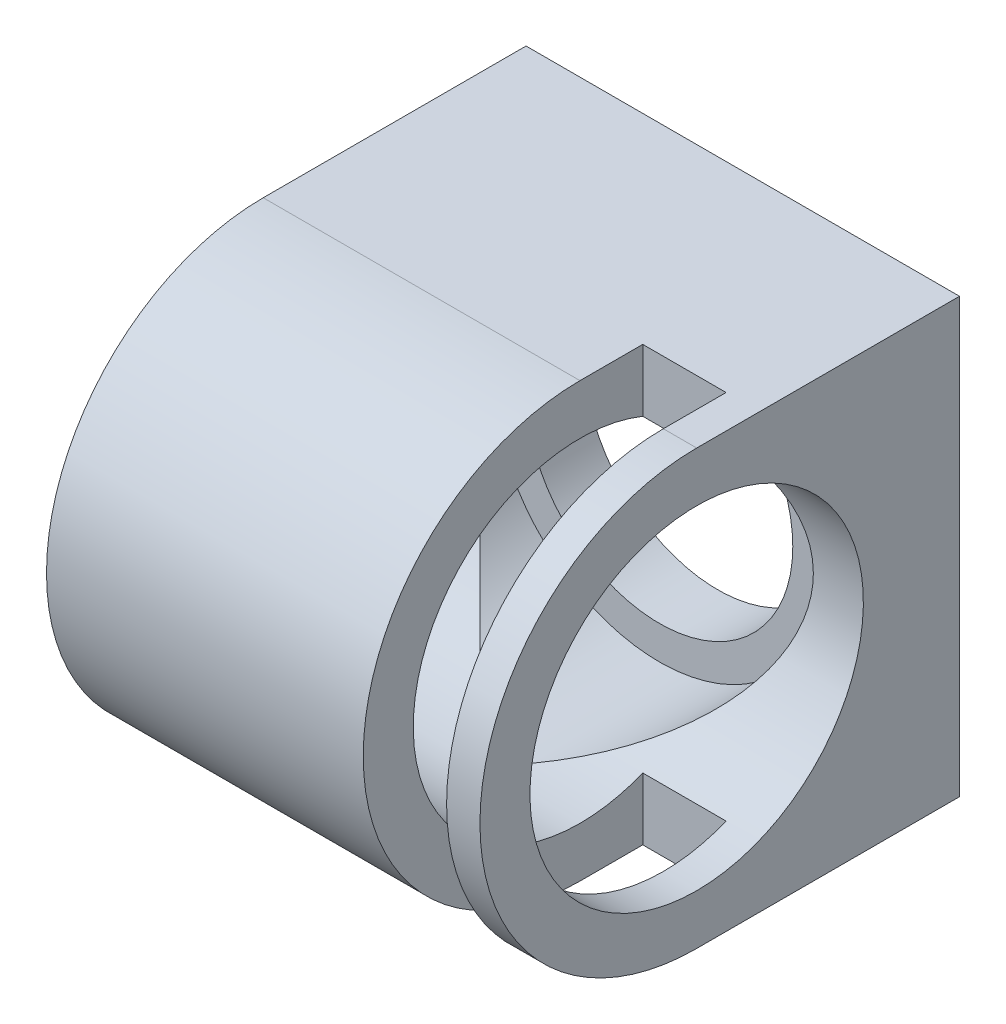
from build123d import *

# Parameters (mm, degrees)
SKETCH3_W           = 52
SKETCH3_H           = 52
BOSS_EXTRUDE1_DEPTH = 10
SKETCH4_R           = 2
CUT_EXTRUDE1_DEPTH  = 10
SKETCH5_R           = 25
CUT_EXTRUDE2_DEPTH  = 3
SKETCH6_R           = 16
CUT_EXTRUDE3_DEPTH  = 38.429934544
SKETCH8_W           = 21.53152206
SKETCH8_H           = 52
BOSS_EXTRUDE2_DEPTH = 52
SKETCH9_R           = 20
CUT_EXTRUDE4_DEPTH  = 21.53152206
BOSS_EXTRUDE3_DEPTH = 52
SKETCH11_R          = 20
CUT_EXTRUDE5_DEPTH  = 52
SKETCH12_W          = 34.659031173
SKETCH12_H          = 60
CUT_EXTRUDE6_DEPTH  = 10


with BuildPart() as part:
    # Sketch3 → Boss-Extrude1 (new body)
    with BuildSketch(Plane.XY):
        Rectangle(SKETCH3_W, SKETCH3_H)
    extrude(amount=BOSS_EXTRUDE1_DEPTH)

    # Sketch4 → Cut-Extrude1 (cut)
    with BuildSketch(Plane(origin=(0, 0, 0), x_dir=(-1, 0, 0), z_dir=(0, 0, -1))):
        with Locations((-21, 21)):
            Circle(SKETCH4_R)
        with Locations(Location((21, 21, 0), (0, 0, 180))):
            Circle(SKETCH4_R)
        with Locations((21, -21)):
            Circle(SKETCH4_R)
        with Locations(Location((-21, -21, 0), (0, 0, 180))):
            Circle(SKETCH4_R)
    extrude(amount=-CUT_EXTRUDE1_DEPTH, mode=Mode.SUBTRACT)

    # Sketch5 → Cut-Extrude2 (cut)
    with BuildSketch(Plane(origin=(0, 0, 0), x_dir=(-1, 0, 0), z_dir=(0, 0, -1))):
        Circle(SKETCH5_R)
    extrude(amount=-CUT_EXTRUDE2_DEPTH, mode=Mode.SUBTRACT)

    # Sketch6 → Cut-Extrude3 (cut, through all)
    with BuildSketch(Plane(origin=(0, 0, 3), x_dir=(-1, 0, 0), z_dir=(0, 0, -1))):
        Circle(SKETCH6_R)
    extrude(amount=-CUT_EXTRUDE3_DEPTH, mode=Mode.SUBTRACT)

    # Sketch8 → Boss-Extrude2 (add)
    with BuildSketch(Plane.ZY.offset(26)):
        with Locations((20.76576103, 0)):
            Rectangle(SKETCH8_W, SKETCH8_H)
    extrude(amount=-BOSS_EXTRUDE2_DEPTH)

    # Sketch9 → Cut-Extrude4 (cut)
    with BuildSketch(Plane.XY.offset(31.53152206)):
        Circle(SKETCH9_R)
    extrude(amount=-CUT_EXTRUDE4_DEPTH, mode=Mode.SUBTRACT)

    # Sketch10 → Boss-Extrude3 (add)
    with BuildSketch(Plane.ZY.offset(26)):
        with BuildLine():
            Line((31.53152206, 26), (31.53152206, -26))
            ThreePointArc((31.53152206, -26), (57.53152206, 0), (31.53152206, 26))
        make_face()
    extrude(amount=-BOSS_EXTRUDE3_DEPTH)

    # Sketch11 → Cut-Extrude5 (cut)
    with BuildSketch(Plane.ZY.offset(26)):
        with Locations(Location((31.53152206, 0, 0), (0, 0, 270))):
            Circle(SKETCH11_R)
    extrude(amount=-CUT_EXTRUDE5_DEPTH, mode=Mode.SUBTRACT)

    # Sketch12 → Cut-Extrude6 (cut)
    with BuildSketch(Plane(origin=(22, 0, 0), x_dir=(0, 0, -1), z_dir=(1, 0, 0))):
        with Locations((-41.329515587, 0)):
            Rectangle(SKETCH12_W, SKETCH12_H)
    extrude(amount=-CUT_EXTRUDE6_DEPTH, mode=Mode.SUBTRACT)


solid = part.part
